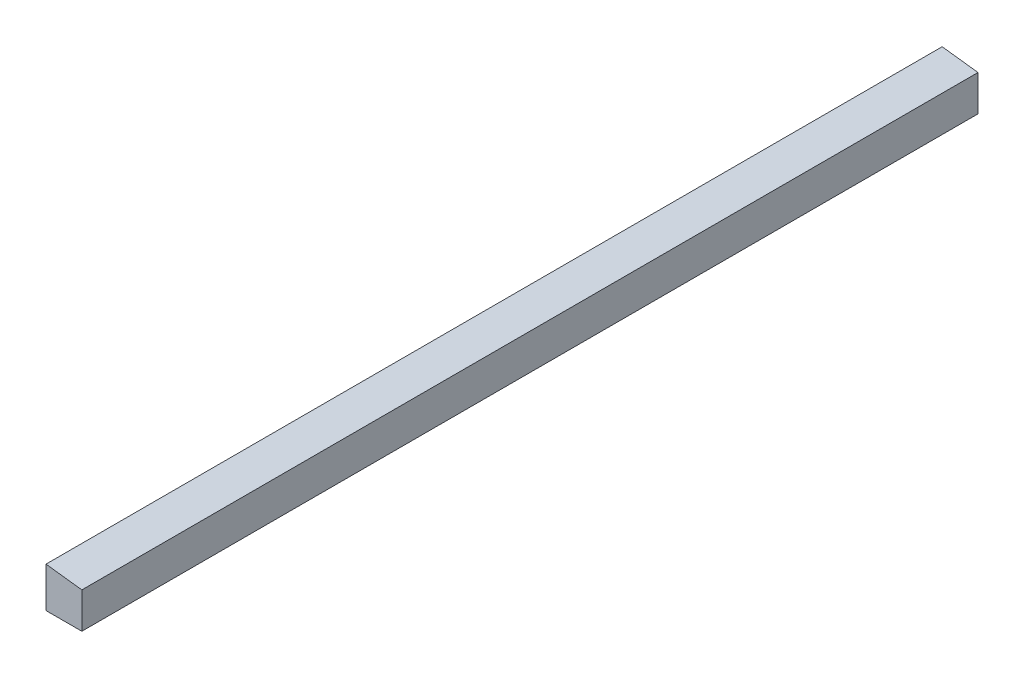
from build123d import *

# Parameters (mm, degrees)
BOSS_EXTRUDE1_DEPTH = 250


with BuildPart() as part:
    # Sketch1 → Boss-Extrude1 (new body)
    with BuildSketch(Plane.XY):
        Polygon((0, 0), (0, 11.227845609), (10, 10), (10, 0), align=None)
    extrude(amount=BOSS_EXTRUDE1_DEPTH)


solid = part.part
